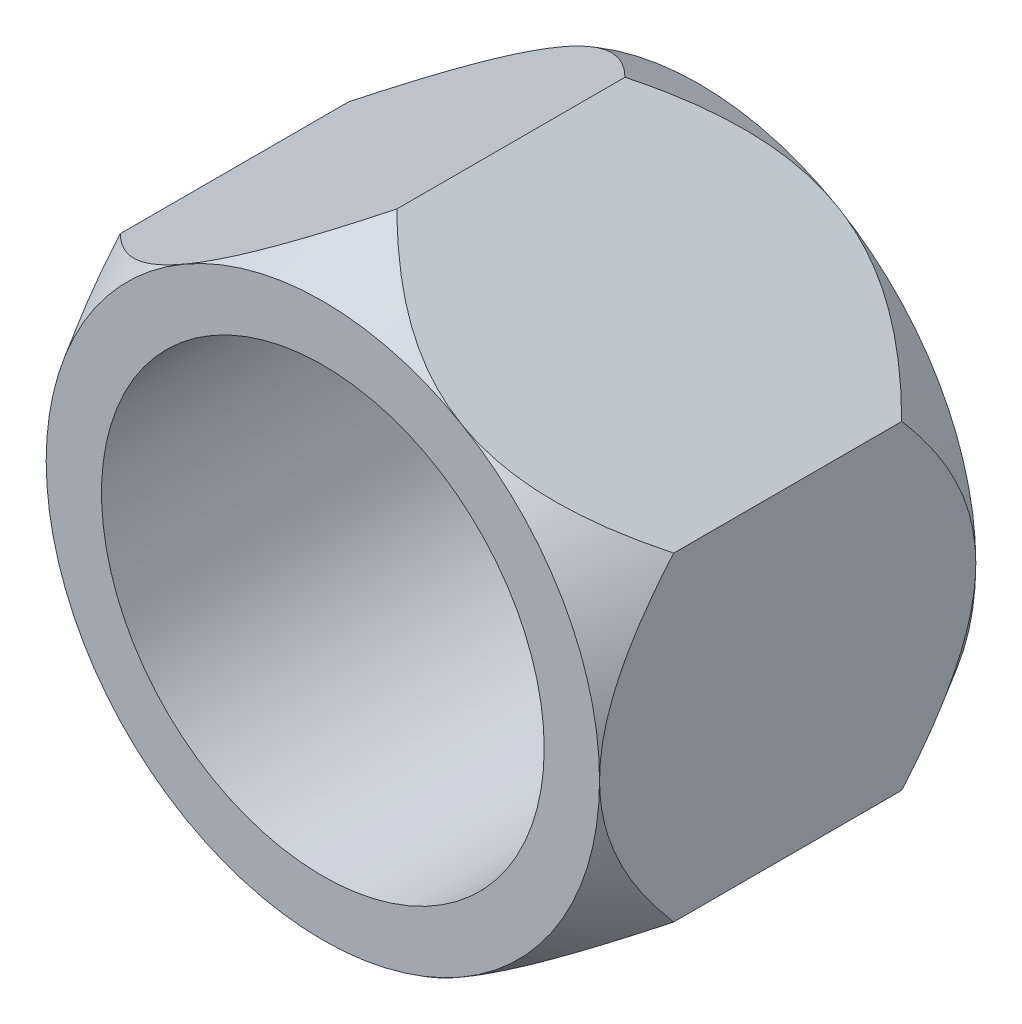
SolidWorks part; units mm, degrees
ref_plane "Front Plane" through (0, 0, 0) normal (0, 0, 1) x (1, 0, 0)
ref_plane "Top Plane" through (0, 0, 0) normal (0, 1, 0) x (1, 0, 0)
ref_plane "Right Plane" through (0, 0, 0) normal (1, 0, 0) x (0, 0, -1)
sketch "Sketch1" plane through (0, 0, 0) normal (0, 0, 1) x (1, 0, 0)
  line L1 (0, 5.7735) -> (-5, 2.8868)
  line L2 (-5, 2.8868) -> (-5, -2.8868)
  line L3 (-5, -2.8868) -> (0, -5.7735)
  line L4 (0, -5.7735) -> (5, -2.8868)
  line L5 (5, -2.8868) -> (5, 2.8868)
  line L6 (5, 2.8868) -> (0, 5.7735)
  circle A0 centre (0, 0) radius 5 construction
  dimension "D1" = 10
extrude "Boss-Extrude1" add sketch "Sketch1" along normal mid plane 6.8
sketch "Sketch2" plane through (0, 0, 3.4) normal (0, 0, 1) x (1, 0, 0)
  line L0 (5, -2.8868) -> (5, 2.8868) construction
  circle A0 centre (0, 0) radius 5
extrude "Cut-Extrude1" cut sketch "Sketch2" against normal blind 6.8 draft 30 flip side to cut
mirror "Mirror1" about plane through (0, 0, 0) normal (0, 0, 1) of "Cut-Extrude1"
sketch "Sketch3" plane through (0, 0, 3.4) normal (0, 0, 1) x (1, 0, 0)
  circle A0 centre (0, 0) radius 4
  dimension "D1" = 8
extrude "Cut-Extrude3" cut sketch "Sketch3" against normal blind 6.8
